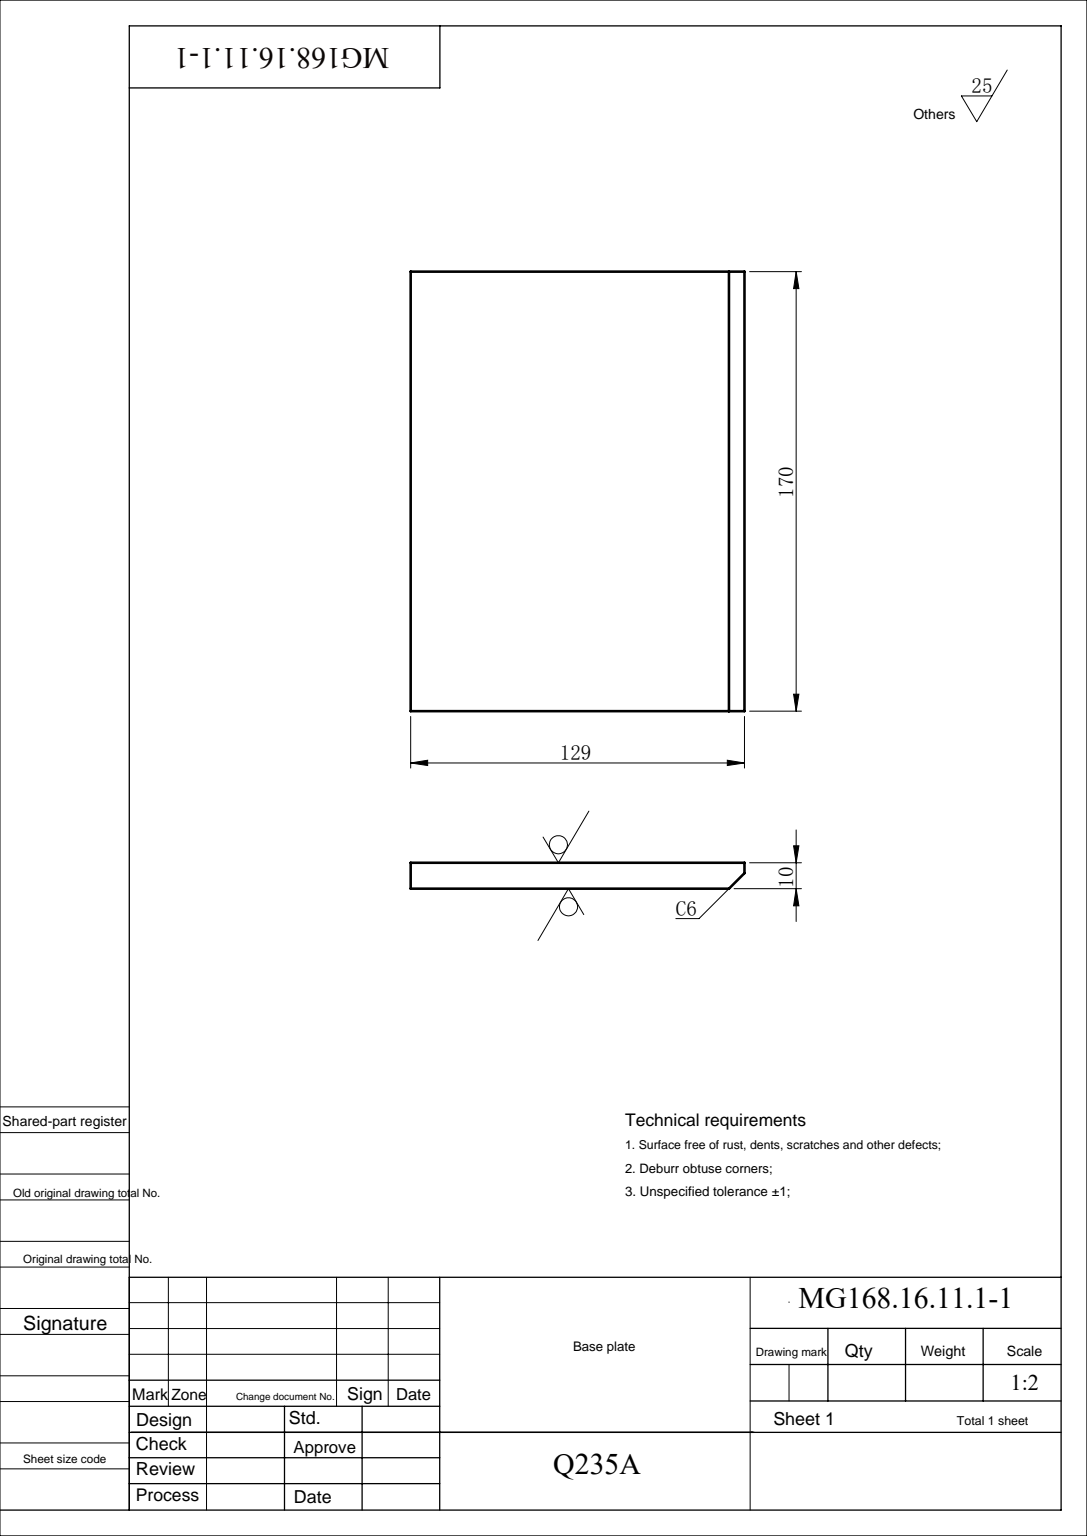
from build123d import *

# Parameters (mm, degrees)
SKETCH1_W           = 129
SKETCH1_H           = 170
BOSS_EXTRUDE1_DEPTH = 5
CHAMFER1_SIZE       = 6


with BuildPart() as part:
    # Sketch1 → Boss-Extrude1 (new, symmetric)
    with BuildSketch(Plane(origin=(0, 0, 0), x_dir=(1, 0, 0), z_dir=(0, 1, 0))):
        with Locations((6.5, 0)):
            Rectangle(SKETCH1_W, SKETCH1_H)
    extrude(amount=BOSS_EXTRUDE1_DEPTH, both=True)

    # Chamfer1
    chamfer1_edges = [part.edges().sort_by_distance(p)[0] for p in [
        (71, 5, 0),
    ]]
    chamfer(chamfer1_edges, length=CHAMFER1_SIZE)


solid = part.part
